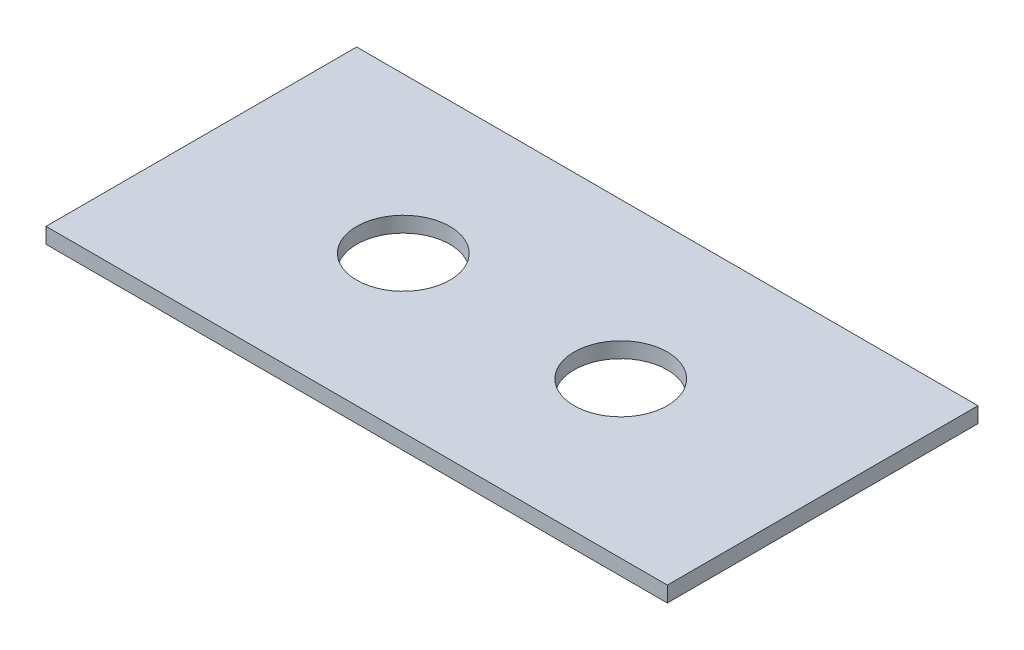
from build123d import *

# Parameters (mm, degrees)
SKETCH1_W           = 20
SKETCH1_H           = 10
SKETCH1_R           = 1.5
BOSS_EXTRUDE1_DEPTH = 0.5


with BuildPart() as part:
    # Sketch1 → Boss-Extrude1 (new body)
    with BuildSketch(Plane(origin=(0, 0, 0), x_dir=(1, 0, 0), z_dir=(0, 1, 0))):
        Rectangle(SKETCH1_W, SKETCH1_H)
        with Locations(Location((-3.5, 0, 0), (0, 0, 270))):
            Circle(SKETCH1_R, mode=Mode.SUBTRACT)
        with Locations(Location((3.5, 0, 0), (0, 0, 90))):
            Circle(SKETCH1_R, mode=Mode.SUBTRACT)
    extrude(amount=BOSS_EXTRUDE1_DEPTH)


solid = part.part
